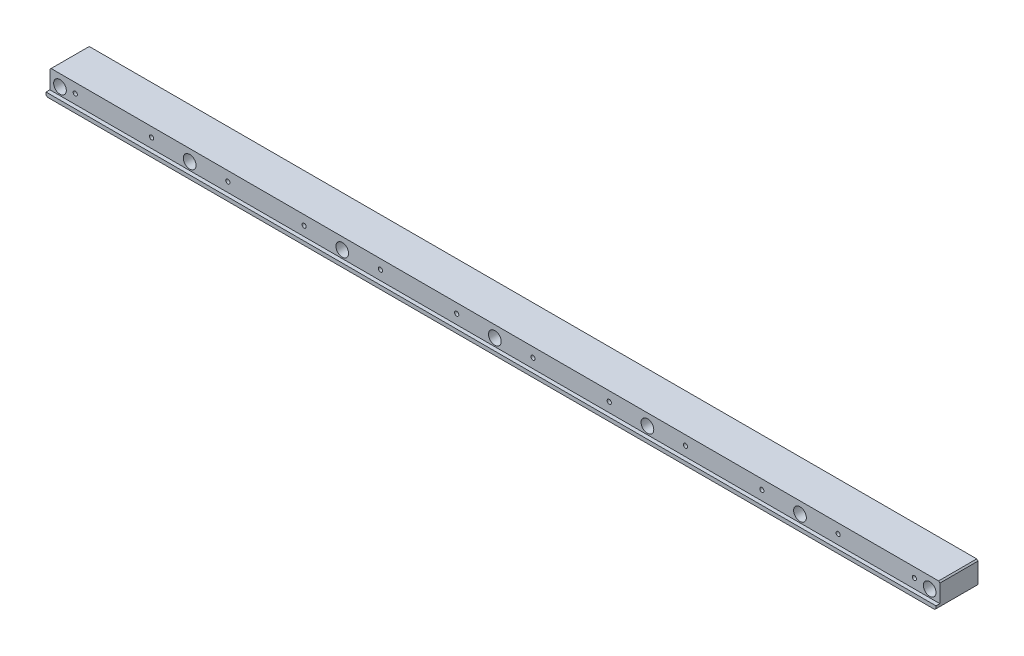
from build123d import *

# Parameters (mm, degrees)
SKETCH1_W                                           = 700
SKETCH1_H                                           = 18
BOSS_EXTRUDE1_DEPTH                                 = 16.5
SKETCH4_W                                           = 700
SKETCH4_H                                           = 15
CUT_EXTRUDE1_DEPTH                                  = 3
M4_TAPPED_HOLE1_D                                   = 3.3
M4_TAPPED_HOLE1_DEPTH                               = 15.5
M4_TAPPED_HOLE1_TIP                                 = 0.991420021
CBORE_FOR_M5_HEX_SOCKET_HEAD_CAP_SCREW1_D           = 5.5
CBORE_FOR_M5_HEX_SOCKET_HEAD_CAP_SCREW1_CBORE_D     = 10
CBORE_FOR_M5_HEX_SOCKET_HEAD_CAP_SCREW1_CBORE_DEPTH = 18
SIZE_MM_DOWEL_HOLE_1_D                              = 8
SIZE_MM_DOWEL_HOLE_1_DEPTH                          = 11
SIZE_MM_DOWEL_HOLE_1_TIP                            = 2.403442476
CHAMFER1_SIZE                                       = 1


with BuildPart() as part:
    # Sketch1 → Boss-Extrude1 (new, symmetric)
    with BuildSketch(Plane.XY):
        Rectangle(SKETCH1_W, SKETCH1_H)
    extrude(amount=BOSS_EXTRUDE1_DEPTH, both=True)

    # Sketch4 → Cut-Extrude1 (cut)
    with BuildSketch(Plane.XY.offset(16.5)):
        with Locations((0, 1.5)):
            Rectangle(SKETCH4_W, SKETCH4_H)
    extrude(amount=-CUT_EXTRUDE1_DEPTH, mode=Mode.SUBTRACT)

    # M4 Tapped Hole1
    with Locations(Plane.XY.offset(13.5)):
        with Locations((330, 1.5), (270, 1.5), (210, 1.5), (150, 1.5), (90, 1.5), (30, 1.5), (-30, 1.5), (-90, 1.5), (-150, 1.5), (-330, 1.5), (-210, 1.5), (-270, 1.5)):
            Hole(M4_TAPPED_HOLE1_D / 2, depth=M4_TAPPED_HOLE1_DEPTH)
            with Locations((0, 0, -(M4_TAPPED_HOLE1_DEPTH + M4_TAPPED_HOLE1_TIP / 2))):  # 118° drill point
                Cone(0, M4_TAPPED_HOLE1_D / 2, M4_TAPPED_HOLE1_TIP, mode=Mode.SUBTRACT)

    # CBORE for M5 Hex Socket Head Cap Screw1 (through all)
    with Locations(Plane.XY.offset(16.5)):
        with Locations((-342, 0), (-240, 0), (-120, 0), (0, 0), (120, 0), (240, 0), (342, 0)):
            CounterBoreHole(CBORE_FOR_M5_HEX_SOCKET_HEAD_CAP_SCREW1_D / 2, CBORE_FOR_M5_HEX_SOCKET_HEAD_CAP_SCREW1_CBORE_D / 2, CBORE_FOR_M5_HEX_SOCKET_HEAD_CAP_SCREW1_CBORE_DEPTH)

    # Size mm dowel hole 1
    with Locations(Plane(origin=(0, 0, -16.5), x_dir=(-1, 0, 0), z_dir=(0, 0, -1))):
        with Locations((-300, 0), (300, 0)):
            Hole(SIZE_MM_DOWEL_HOLE_1_D / 2, depth=SIZE_MM_DOWEL_HOLE_1_DEPTH)
            with Locations((0, 0, -(SIZE_MM_DOWEL_HOLE_1_DEPTH + SIZE_MM_DOWEL_HOLE_1_TIP / 2))):  # 118° drill point
                Cone(0, SIZE_MM_DOWEL_HOLE_1_D / 2, SIZE_MM_DOWEL_HOLE_1_TIP, mode=Mode.SUBTRACT)

    # Chamfer1
    chamfer1_edges = [part.edges().sort_by_distance(p)[0] for p in [
        (-350, 9, -1.5),
        (350, 9, -1.5),
        (350, -9, 0),
        (-350, -9, 0),
    ]]
    chamfer(chamfer1_edges, length=CHAMFER1_SIZE)


solid = part.part
